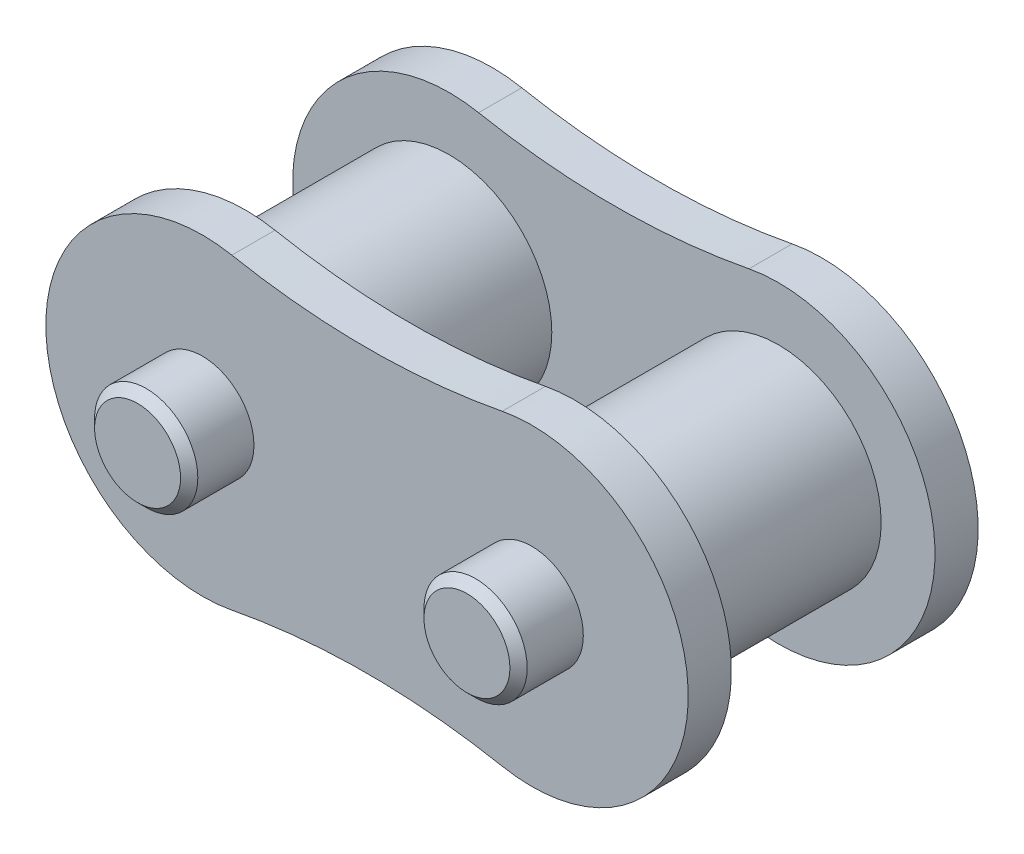
SolidWorks part; units mm, degrees
ref_plane "前视基准面" through (0, 0, 0) normal (0, 0, 1) x (1, 0, 0)
ref_plane "上视基准面" through (0, 0, 0) normal (0, 1, 0) x (1, 0, 0)
ref_plane "右视基准面" through (0, 0, 0) normal (1, 0, 0) x (0, 0, -1)
sketch "草图1" plane through (0, 0, 0) normal (0, 0, 1) x (1, 0, 0)
  line L0 (-6.35, 0) -> (6.35, 0) construction
  line L1 (0, 5.4315) -> (0, -5.4315) construction
  line L2 (6.35, 0) -> (17.53, 0) construction
  line L3 (17.53, 0) -> (25.38, 0) construction
  circle A0 centre (-6.35, 0) radius 6.035
  circle A1 centre (6.35, 0) radius 6.035
  circle A2 centre (0, 33.1055) radius 27.674
  circle A3 centre (0, -33.1055) radius 27.674
  circle A4 centre (-6.35, 0) radius 3.96
  circle A5 centre (6.35, 0) radius 3.96
  circle A6 centre (-6.35, 0) radius 1.99
  circle A7 centre (6.35, 0) radius 1.99
sketch "草图2" plane through (0, 0, 0) normal (0, 0, 1) x (1, 0, 0)
  circle A0 centre (6.35, 0) radius 3.96 construction
  circle A1 centre (-6.35, 0) radius 3.96 construction
  circle A2 centre (6.35, 0) radius 3.96
  circle A3 centre (-6.35, 0) radius 3.96
extrude "拉伸1" add sketch "草图2" along normal mid plane 7.85
sketch "草图3" plane through (0, 0, 3.925) normal (0, 0, 1) x (1, 0, 0)
  circle A0 centre (-6.35, 0) radius 6.035 construction
  arc A1 (-5.2131, 5.927) -> (-5.2131, -5.927) centre (-6.35, 0) ccw
  circle A2 centre (6.35, 0) radius 6.035 construction
  arc A3 (5.2131, -5.927) -> (5.2131, 5.927) centre (6.35, 0) ccw
  circle A4 centre (0, 33.1055) radius 27.674 construction
  arc A5 (-5.2131, 5.927) -> (5.2131, 5.927) centre (0, 33.1055) ccw
  circle A6 centre (0, -33.1055) radius 27.674 construction
  arc A7 (5.2131, -5.927) -> (-5.2131, -5.927) centre (0, -33.1055) ccw
extrude "拉伸2" add sketch "草图3" along normal blind 1.665
sketch "草图4" plane through (0, 0, 5.59) normal (0, 0, 1) x (1, 0, 0)
  circle A0 centre (6.35, 0) radius 1.99 construction
  circle A1 centre (-6.35, 0) radius 1.99 construction
  circle A2 centre (6.35, 0) radius 1.99
  circle A3 centre (-6.35, 0) radius 1.99
extrude "拉伸3" add sketch "草图4" along normal blind 2.4975
chamfer "倒角1" distance 0.333 angle 45 2 edges at (8.34, 0, 8.0875) (-4.36, 0, 8.0875)
mirror "镜向1" about plane through (0, 0, 0) normal (0, 0, 1) of "拉伸2", "倒角1", "拉伸3"
equation "\"D1@拉伸2\" = (  \"b2@草图1\" - \"D1@拉伸1\" )  / 2"
equation "\"D1@拉伸3\" = \"D1@拉伸2\" * 1.5"
equation "\"D1@倒角1\" = \"D1@拉伸2\" / 5"
equation "\"D1@拉伸1\"= \"b1@草图1\""
equation "\"h3@草图1\" = \"h2@草图1\" * 0.9"
